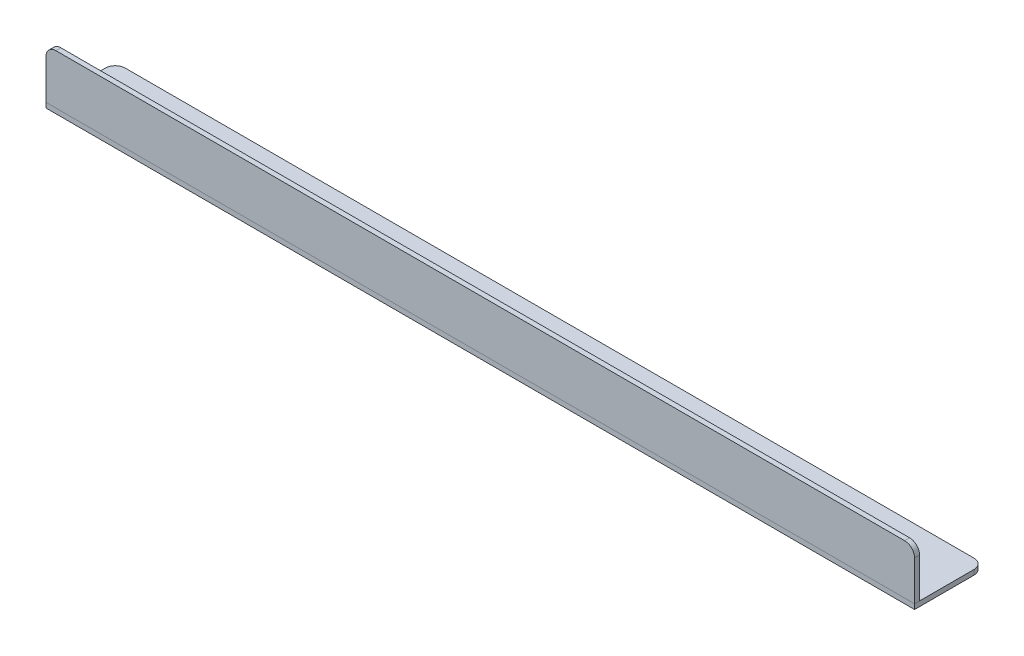
SolidWorks part; units mm, degrees
ref_plane "前视基准面" through (0, 0, 0) normal (0, 0, 1) x (1, 0, 0)
ref_plane "上视基准面" through (0, 0, 0) normal (0, 1, 0) x (1, 0, 0)
ref_plane "右视基准面" through (0, 0, 0) normal (1, 0, 0) x (0, 0, -1)
other "Configuration Table"
sketch "草图1" plane through (0, 0, 0) normal (0, 1, 0) x (1, 0, 0)
  line L1 (-873.75, 69.7) -> (873.75, 69.7)
  line L2 (-873.75, 69.7) -> (-873.75, -69.7)
  line L3 (-873.75, -69.7) -> (873.75, -69.7)
  line L4 (873.75, 69.7) -> (873.75, -69.7)
  line L5 (-873.75, 69.7) -> (873.75, -69.7) construction
  line L6 (-873.75, -69.7) -> (873.75, 69.7) construction
  point P0 (0, 0)
  dimension "D1" = 1747.5
  dimension "D2" = 139.4
extrude "凸台-拉伸1" add sketch "草图1" along normal blind 10
sketch "草图2" plane through (0, 0, 69.7) normal (0, 0, 1) x (1, 0, 0)
  line L0 (873.75, 10) -> (873.75, 0) construction
  line L1 (-873.75, 10) -> (873.75, 10)
  line L2 (-873.75, 10) -> (-873.75, 110)
  line L3 (-873.75, 110) -> (873.75, 110)
  line L4 (873.75, 10) -> (873.75, 110)
  dimension "D1" = 100
extrude "凸台-拉伸2" add sketch "草图2" against normal blind 10 separate body
sketch "草图3" plane through (0, 0, 0) normal (1, 0, 0) x (0, 0, -1)
  line L0 (0, 10) -> (-59.7, 60)
  line L1 (-69.7, 10) -> (69.7, 10) construction
  line L2 (-59.7, 10) -> (-59.7, 110) construction
  line L3 (-59.7, 60) -> (-59.7, 10)
  line L4 (-59.7, 10) -> (0, 10)
extrude "凸台-拉伸3" add sketch "草图3" along normal mid plane 10 separate body
fillet "圆角1" radius 20 2 edges at (873.75, 110, 64.7) (-873.75, 110, 64.7)
fillet "圆角2" radius 20 2 edges at (-873.75, 5, -69.7) (873.75, 5, -69.7)
